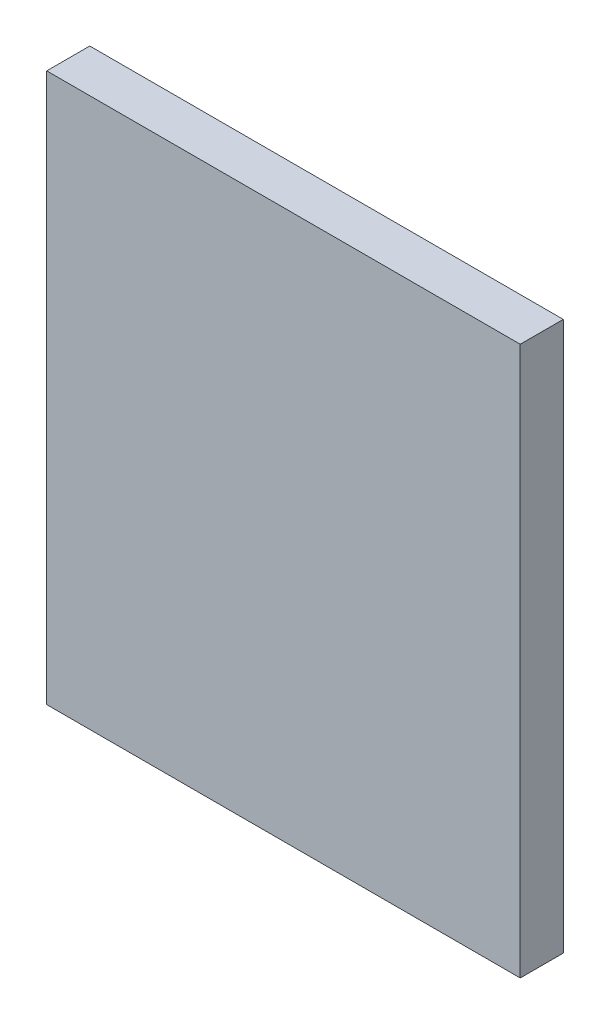
SolidWorks part; units mm, degrees
material "Q235"
ref_plane "Front Plane" through (0, 0, 0) normal (0, 0, 1) x (1, 0, 0)
ref_plane "Top Plane" through (0, 0, 0) normal (0, 1, 0) x (1, 0, 0)
ref_plane "Right Plane" through (0, 0, 0) normal (1, 0, 0) x (0, 0, -1)
sketch "Sketch1" plane through (0, 0, 0) normal (0, 0, 1) x (1, 0, 0)
  line L1 (0, 0) -> (440, 0)
  line L2 (0, 0) -> (0, 510)
  line L3 (0, 510) -> (440, 510)
  line L4 (440, 0) -> (440, 510)
  dimension "D1" = 510
  dimension "D2" = 440
extrude "Boss-Extrude1" add sketch "Sketch1" along normal blind 40
